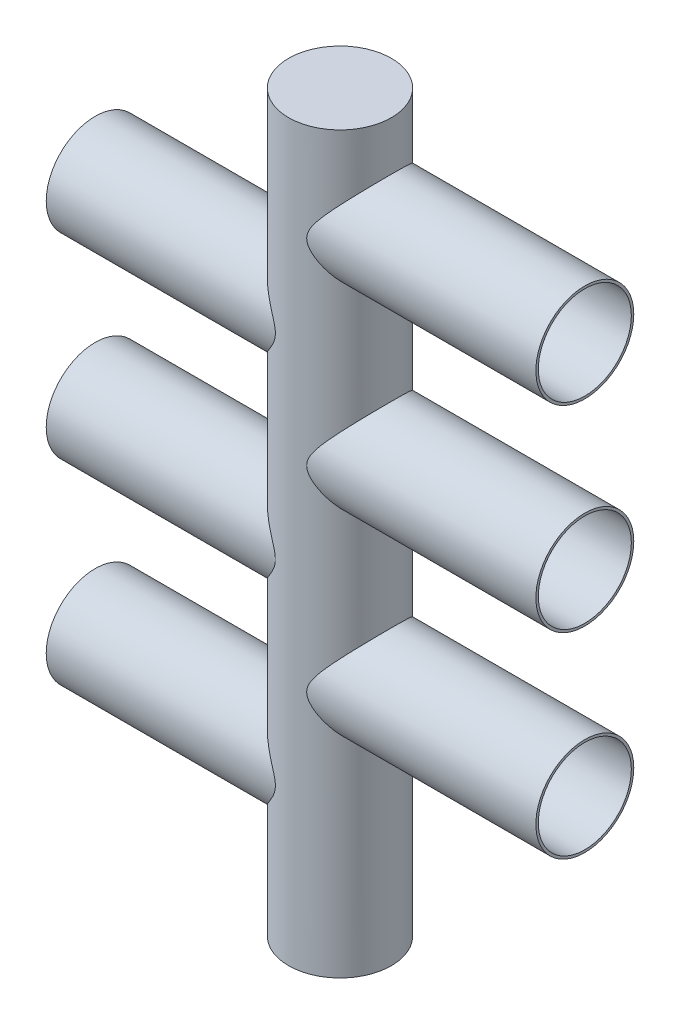
from build123d import *

# Parameters (mm, degrees)
SKETCH2_R                = 10.5
SKETCH2_R_2              = 10
BOSS_EXTRUDE1_DEPTH      = 150
BOSS_EXTRUDE2_START      = -5
SKETCH3_R                = 10.5
BOSS_EXTRUDE2_DEPTH      = 5
BOSS_EXTRUDE3_REACH      = 127.978
BOSS_EXTRUDE3_END_RADIUS = 10.5
SKETCH5_R                = 10
SKETCH5_R_2              = 9.5
BOSS_EXTRUDE4_REACH      = 166.348
BOSS_EXTRUDE4_END_RADIUS = 10.5
SKETCH4_R                = 10
SKETCH4_R_2              = 9.5
SKETCH7_R                = 9.5
CUT_EXTRUDE3_DEPTH       = 50
SKETCH8_R                = 9.5
CUT_EXTRUDE4_DEPTH       = 46


with BuildPart() as part:
    # Sketch2 → Boss-Extrude1 (new body)
    with BuildSketch(Plane(origin=(0, -41.034088034, 0), x_dir=(1, 0, 0), z_dir=(0, 1, 0))):
        with Locations(Location((0, 0, 0), (0, 0, 270))):
            Circle(SKETCH2_R)
        with Locations(Location((0, 0, 0), (0, 0, 270))):
            Circle(SKETCH2_R_2, mode=Mode.SUBTRACT)
    extrude(amount=BOSS_EXTRUDE1_DEPTH)

    # Sketch3 → Boss-Extrude2 (add)
    with BuildSketch(Plane(origin=(0, 108.965911966, 0), x_dir=(1, 0, 0), z_dir=(0, 1, 0)).offset(BOSS_EXTRUDE2_START)):
        with Locations(Location((0, 0, 0), (0, 0, 270))):
            Circle(SKETCH3_R)
    extrude(amount=BOSS_EXTRUDE2_DEPTH)

    # Boss-Extrude3: up to this cylinder (the profile starts outside it)
    boss_extrude3_end = Plane(origin=(0, 28.965912, 0), z_dir=(0, -1, 0)) * Cylinder(BOSS_EXTRUDE3_END_RADIUS, 357.956, mode=Mode.PRIVATE)
    # Sketch5 → Boss-Extrude3 (add, up to the surface)
    with BuildSketch(Plane(origin=(-50, 68.965911966, 0), x_dir=(0, 0, 1), z_dir=(-1, 0, 0)), mode=Mode.PRIVATE) as boss_extrude3_sk1:
        Circle(SKETCH5_R)
        Circle(SKETCH5_R_2, mode=Mode.SUBTRACT)
    boss_extrude3_tool1 = extrude(boss_extrude3_sk1.sketch, amount=-BOSS_EXTRUDE3_REACH, mode=Mode.PRIVATE) - boss_extrude3_end
    add(boss_extrude3_tool1.solids().sort_by_distance((-50, 68.965912, -9.717157))[0])
    # Sketch5 → Boss-Extrude3 (add, up to the surface)
    with BuildSketch(Plane(origin=(-50, 68.965911966, 0), x_dir=(0, 0, 1), z_dir=(-1, 0, 0)), mode=Mode.PRIVATE) as boss_extrude3_sk2:
        with Locations((0, -40)):
            Circle(SKETCH5_R)
        with Locations((0, -40)):
            Circle(SKETCH5_R_2, mode=Mode.SUBTRACT)
    boss_extrude3_tool2 = extrude(boss_extrude3_sk2.sketch, amount=-BOSS_EXTRUDE3_REACH, mode=Mode.PRIVATE) - boss_extrude3_end
    add(boss_extrude3_tool2.solids().sort_by_distance((-50, 28.965912, -9.717157))[0])
    # Sketch5 → Boss-Extrude3 (add, up to the surface)
    with BuildSketch(Plane(origin=(-50, 68.965911966, 0), x_dir=(0, 0, 1), z_dir=(-1, 0, 0)), mode=Mode.PRIVATE) as boss_extrude3_sk3:
        with Locations((0, -80)):
            Circle(SKETCH5_R)
        with Locations((0, -80)):
            Circle(SKETCH5_R_2, mode=Mode.SUBTRACT)
    boss_extrude3_tool3 = extrude(boss_extrude3_sk3.sketch, amount=-BOSS_EXTRUDE3_REACH, mode=Mode.PRIVATE) - boss_extrude3_end
    add(boss_extrude3_tool3.solids().sort_by_distance((-50, -11.034088, -9.717157))[0])

    # Boss-Extrude4: up to this cylinder (the profile starts outside it)
    boss_extrude4_end = Plane(origin=(0, 48.8468315, 0), z_dir=(0, -1, 0)) * Cylinder(BOSS_EXTRUDE4_END_RADIUS, 434.934161, mode=Mode.PRIVATE)
    # Sketch4 → Boss-Extrude4 (add, up to the surface)
    with BuildSketch(Plane(origin=(50, 88.965911966, 0), x_dir=(0, 0, -1), z_dir=(1, 0, 0)), mode=Mode.PRIVATE) as boss_extrude4_sk1:
        Circle(SKETCH4_R)
        Circle(SKETCH4_R_2, mode=Mode.SUBTRACT)
    boss_extrude4_tool1 = extrude(boss_extrude4_sk1.sketch, amount=-BOSS_EXTRUDE4_REACH, mode=Mode.PRIVATE) - boss_extrude4_end
    add(boss_extrude4_tool1.solids().sort_by_distance((50, 88.965912, 9.717157))[0])
    # Sketch4 → Boss-Extrude4 (add, up to the surface)
    with BuildSketch(Plane(origin=(50, 88.965911966, 0), x_dir=(0, 0, -1), z_dir=(1, 0, 0)), mode=Mode.PRIVATE) as boss_extrude4_sk2:
        with Locations((0, -40.184187959)):
            Circle(SKETCH4_R)
        with Locations((0, -40.184187959)):
            Circle(SKETCH4_R_2, mode=Mode.SUBTRACT)
    boss_extrude4_tool2 = extrude(boss_extrude4_sk2.sketch, amount=-BOSS_EXTRUDE4_REACH, mode=Mode.PRIVATE) - boss_extrude4_end
    add(boss_extrude4_tool2.solids().sort_by_distance((50, 48.781724, 9.717157))[0])
    # Sketch4 → Boss-Extrude4 (add, up to the surface)
    with BuildSketch(Plane(origin=(50, 88.965911966, 0), x_dir=(0, 0, -1), z_dir=(1, 0, 0)), mode=Mode.PRIVATE) as boss_extrude4_sk3:
        with Locations((0, -80.238160601)):
            Circle(SKETCH4_R)
        with Locations((0, -80.238160601)):
            Circle(SKETCH4_R_2, mode=Mode.SUBTRACT)
    boss_extrude4_tool3 = extrude(boss_extrude4_sk3.sketch, amount=-BOSS_EXTRUDE4_REACH, mode=Mode.PRIVATE) - boss_extrude4_end
    add(boss_extrude4_tool3.solids().sort_by_distance((50, 8.727751, 9.717157))[0])

    # Sketch7 → Cut-Extrude3 (cut)
    with BuildSketch(Plane(origin=(50, 88.965911966, 0), x_dir=(0, 0, -1), z_dir=(1, 0, 0))):
        Circle(SKETCH7_R)
        with Locations((0, -40.184187959)):
            Circle(SKETCH7_R)
        with Locations((0, -80.238160601)):
            Circle(SKETCH7_R)
    extrude(amount=-CUT_EXTRUDE3_DEPTH, mode=Mode.SUBTRACT)

    # Sketch8 → Cut-Extrude4 (cut)
    with BuildSketch(Plane(origin=(-50, 68.965911966, 0), x_dir=(0, 0, 1), z_dir=(-1, 0, 0))):
        Circle(SKETCH8_R)
        with Locations((0, -40)):
            Circle(SKETCH8_R)
        with Locations((0, -80)):
            Circle(SKETCH8_R)
    extrude(amount=-CUT_EXTRUDE4_DEPTH, mode=Mode.SUBTRACT)


solid = part.part
